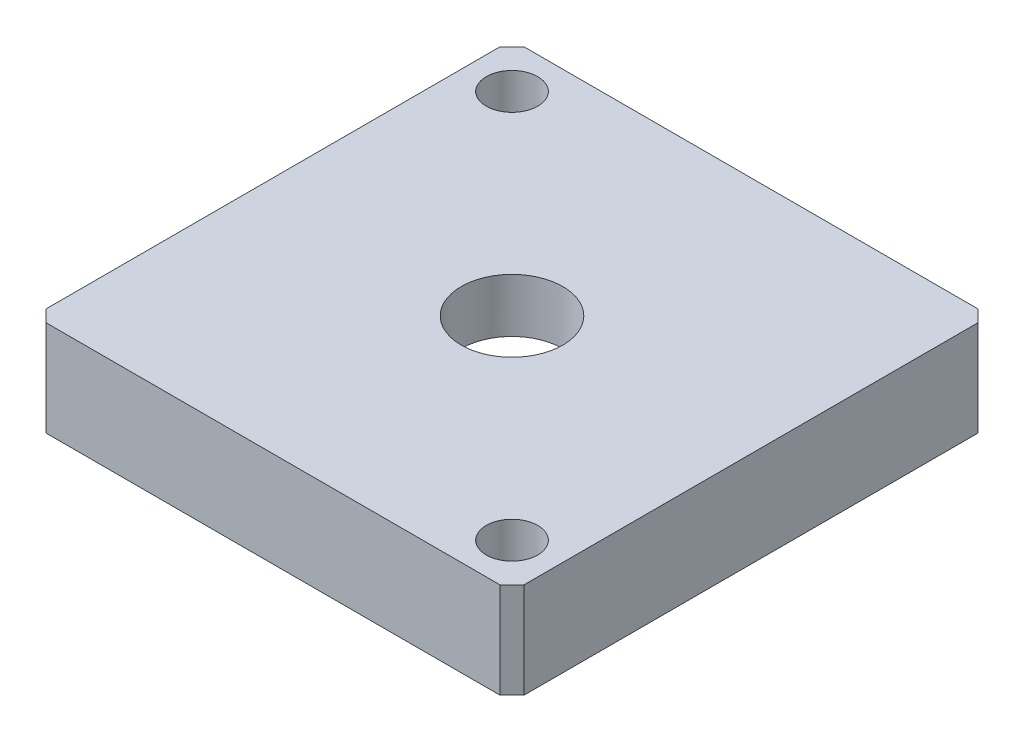
from build123d import *

# Parameters (mm, degrees)
SKETCH1_W           = 40
SKETCH1_H           = 40
BOSS_EXTRUDE1_DEPTH = 8
CHAMFER1_SIZE       = 1
SKETCH2_R           = 15.5
CUT_EXTRUDE1_DEPTH  = 3.5
SKETCH3_R           = 4.25
CUT_EXTRUDE2_DEPTH  = 30.393876913
SKETCH4_R           = 2.15
CUT_EXTRUDE3_DEPTH  = 10


with BuildPart() as part:
    # Sketch1 → Boss-Extrude1 (new body)
    with BuildSketch(Plane(origin=(0, 0, 0), x_dir=(1, 0, 0), z_dir=(0, 1, 0))):
        Rectangle(SKETCH1_W, SKETCH1_H)
    extrude(amount=BOSS_EXTRUDE1_DEPTH)

    # Chamfer1
    chamfer1_edges = [part.edges().sort_by_distance(p)[0] for p in [
        (20, 4, 20),
        (-20, 4, 20),
        (-20, 4, -20),
        (20, 4, -20),
    ]]
    chamfer(chamfer1_edges, length=CHAMFER1_SIZE)

    # Sketch2 → Cut-Extrude1 (cut)
    with BuildSketch(Plane.XZ):
        with Locations(Location((0, 0, 0), (0, 0, 270))):
            Circle(SKETCH2_R)
    extrude(amount=-CUT_EXTRUDE1_DEPTH, mode=Mode.SUBTRACT)

    # Sketch3 → Cut-Extrude2 (cut, through all)
    with BuildSketch(Plane(origin=(0, 8, 0), x_dir=(1, 0, 0), z_dir=(0, 1, 0))):
        with Locations(Location((0, 0, 0), (0, 0, 270))):
            Circle(SKETCH3_R)
    extrude(amount=-CUT_EXTRUDE2_DEPTH, mode=Mode.SUBTRACT)

    # Sketch4 → Cut-Extrude3 (cut)
    with BuildSketch(Plane.XZ):
        with Locations(Location((16.263455967, 16.263455967, 0), (0, 0, 270))):
            Circle(SKETCH4_R)
        with Locations(Location((-16.263455967, -16.263455967, 0), (0, 0, 270))):
            Circle(SKETCH4_R)
    extrude(amount=-CUT_EXTRUDE3_DEPTH, mode=Mode.SUBTRACT)


solid = part.part
